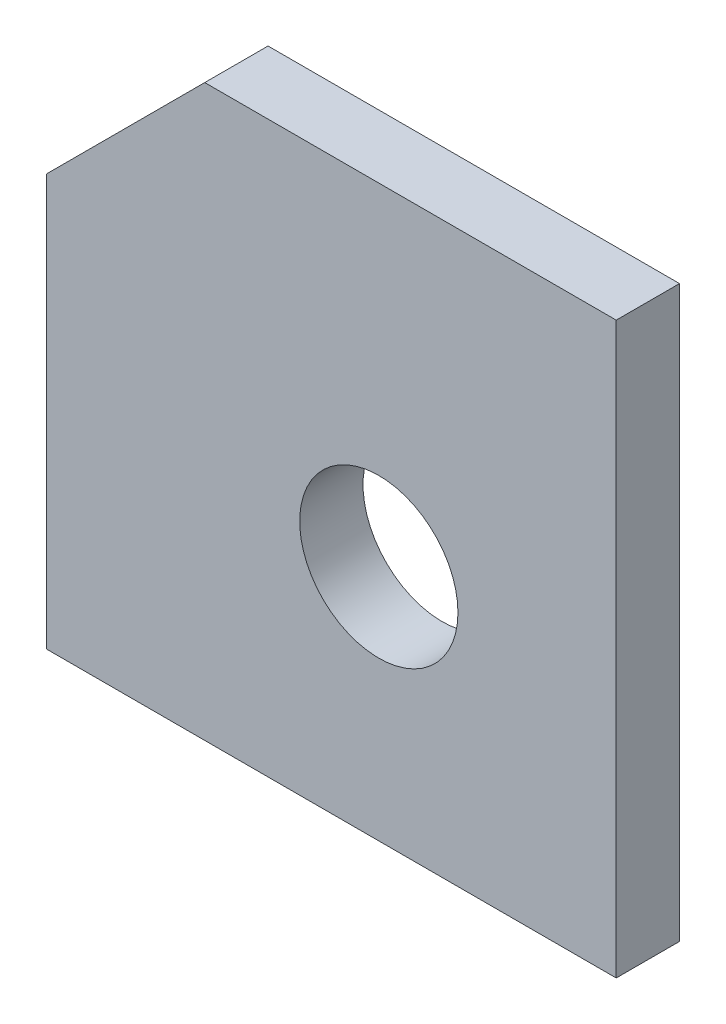
from build123d import *

# Parameters (mm, degrees)
SKETCH_1_W              = 36
SKETCH_1_H              = 36
EXTRUDE_1_DEPTH         = 4
CHAMFER_1_SIZE          = 10
HOLE_WIZARD_10_0_10_1_D = 10


with BuildPart() as part:
    # 草图1 → 凸台-拉伸1 (new body)
    with BuildSketch(Plane.XY):
        with Locations((18, 18)):
            Rectangle(SKETCH_1_W, SKETCH_1_H)
    extrude(amount=EXTRUDE_1_DEPTH)

    # 倒角1
    chamfer_1_edges = [part.edges().sort_by_distance(p)[0] for p in [
        (0, 36, 2),
    ]]
    chamfer(chamfer_1_edges, length=CHAMFER_1_SIZE)

    # Ø10.0 (10) 直径孔1 (through all)
    with Locations(Plane.XY.offset(4)):
        with Locations((21, 15)):
            Hole(HOLE_WIZARD_10_0_10_1_D / 2)


solid = part.part
